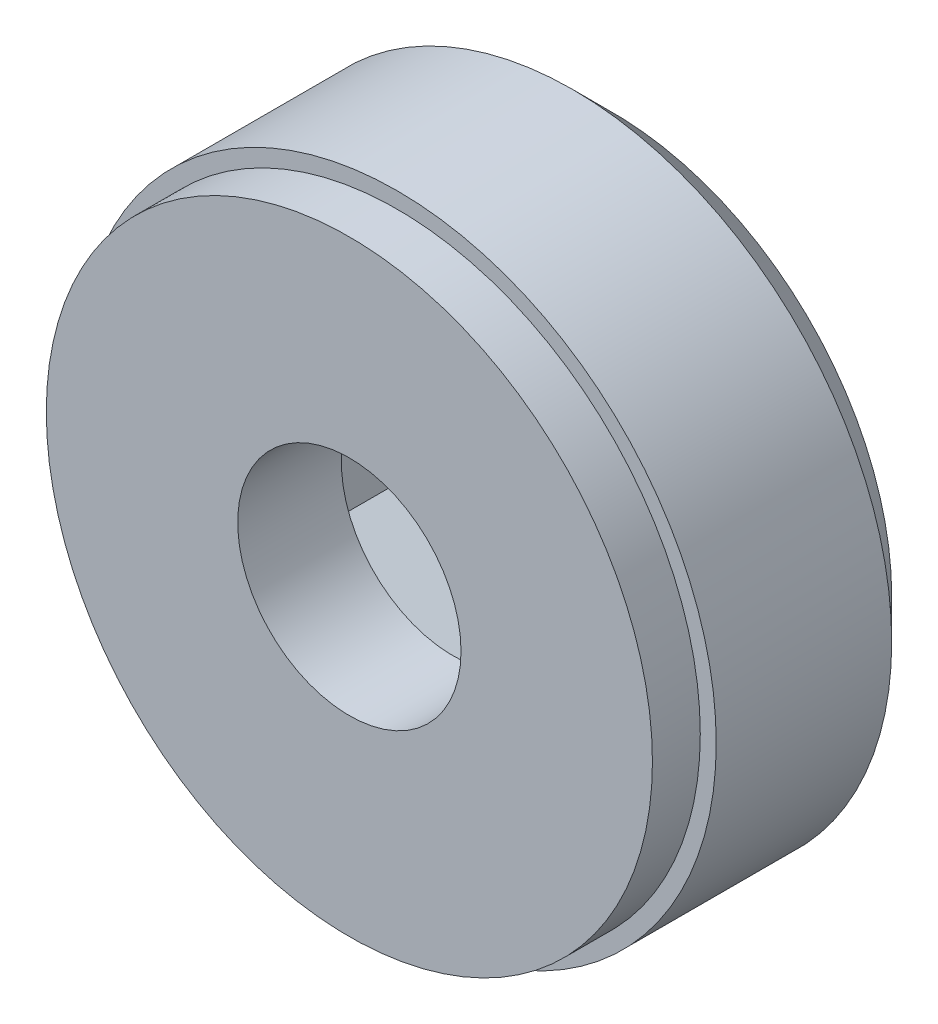
SolidWorks part; units mm, degrees
ref_plane "Front Plane" through (0, 0, 0) normal (0, 0, 1) x (1, 0, 0)
ref_plane "Top Plane" through (0, 0, 0) normal (0, 1, 0) x (1, 0, 0)
ref_plane "Right Plane" through (0, 0, 0) normal (1, 0, 0) x (0, 0, -1)
sketch "Sketch1" plane through (0, 0, 0) normal (0, 0, 1) x (1, 0, 0)
  circle A0 centre (0, 0) radius 40
  dimension "D1" = 80
extrude "Boss-Extrude1" add sketch "Sketch1" along normal blind 33
sketch "Sketch2" plane through (0, 0, 33) normal (0, 0, 1) x (1, 0, 0)
  circle A0 centre (0, 0) radius 38
  circle A1 centre (0, 0) radius 40 construction
  circle A2 centre (0, 0) radius 40
  dimension "D1" = 76
extrude "Cut-Extrude1" cut sketch "Sketch2" against normal blind 6
chamfer "Chamfer1" distance 5 angle 45 1 edges at (40, 0, 0)
sketch "Sketch3" plane through (0, 0, 33) normal (0, 0, 1) x (1, 0, 0)
  circle A0 centre (0, 0) radius 14
  dimension "D1" = 28
extrude "Cut-Extrude2" cut sketch "Sketch3" against normal blind 13
sketch "Sketch4" plane through (0, 0, 0) normal (0, 0, -1) x (-1, 0, 0)
  line L0 (0, 0) -> (0, 29.888) construction
  line L1 (-19.5, -11.2583) -> (0, -22.5167)
  line L2 (0, -22.5167) -> (19.5, -11.2583)
  line L3 (19.5, -11.2583) -> (19.5, 11.2583)
  line L4 (19.5, 11.2583) -> (0, 22.5167)
  line L5 (0, 22.5167) -> (-19.5, 11.2583)
  line L6 (-19.5, 11.2583) -> (-19.5, -11.2583)
  circle A0 centre (0, 0) radius 19.5 construction
  dimension "D1" = 39
extrude "Cut-Extrude3" cut sketch "Sketch4" against normal blind 20
